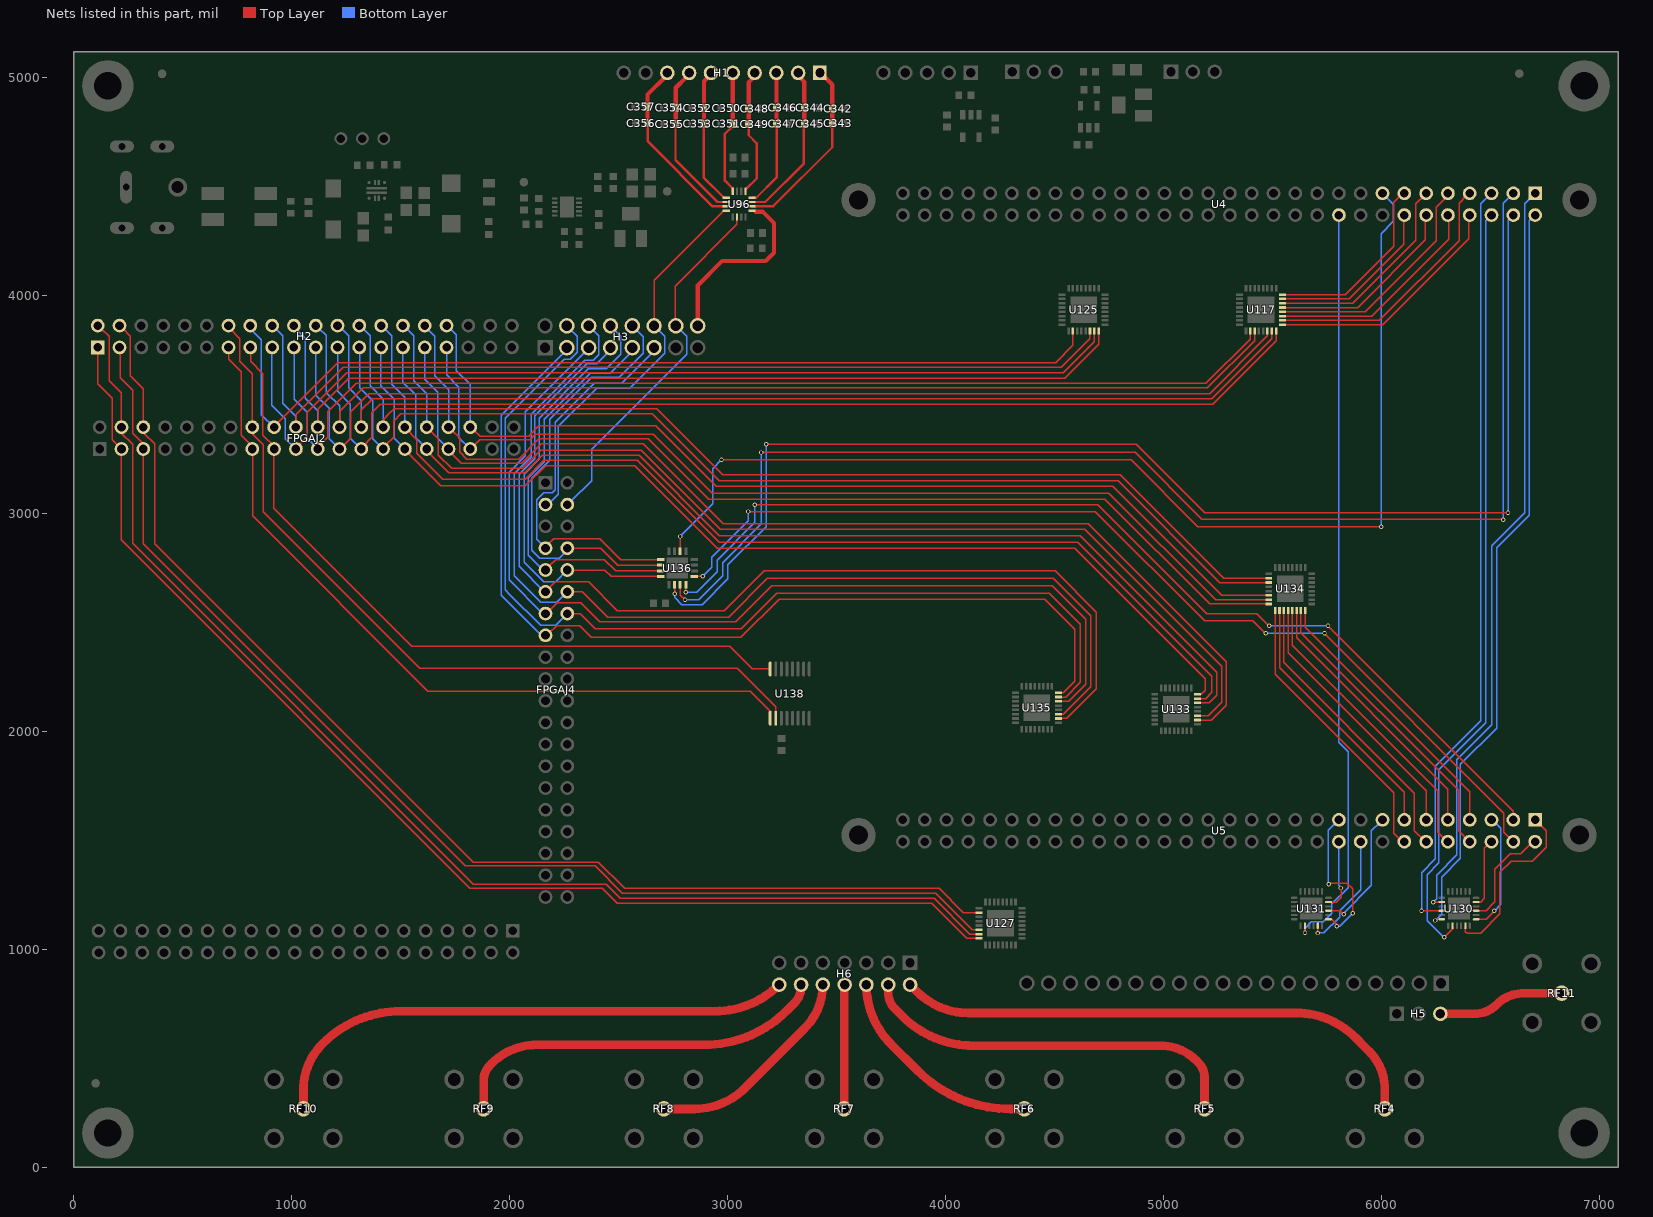
[diagram p0: the nets of this part, all layers, seen from the top]
# Altium PCB MISC82799.PcbDoc (part 2 of 5)
Units mil, origin at the board's own origin, x right, y up, seen from the top; angles counter-clockwise.
Board outline 7086.61 x 5118.11 mil, 4 copper layers (Top Layer, GND, POWER, Bottom Layer); 95 components, 232 nets, 857 pads, 1291 vias.

## Via types
v1: diameter 20, hole 12, Top Layer to Bottom Layer, 1291 vias

## Nets (pads, with @x,y where several pads share a name; then routed paths per layer and width w, separated by ;. In a path a pad name is that pad's centre, name@x,y a point inside that pad or via, vN(x,y) a via of type N, cw(c..) or ccw(c..) an arc to the next point about the centre after c; other vN are vias at no path point) (continued)
A_D_C4: U4.20 U131.8 | length 3458.9
  Top Layer w6: v1(5648.5,1075.5) U131.8@5648.5,1108.26
  Bottom Layer w6: v1@5649,1079 5649,1097 5678,1126 5732,1126 5772,1166 5772,1208 5847,1283 5847,1355 ; U4.20@5804.35,4367.81 5804.35,1949.65 5847,1907 5847,1355 ; 5847,1349 5847,1355
A_D_C5: U5.18 U131.11 | length 549.7
  Top Layer w6: v1(5707.5,1074.5) U131.11@5707.5,1108.26
  Bottom Layer w6: v1@5708,1075 5735,1075 5807,1147 5807,1177 5904.35,1274.35 U5.18@5904.35,1493.8
A_D_C6: U5.19 U131.13 | length 704.4
  Top Layer w6: U131.13@5756.74,1137.8 5772.2,1137.8 5794,1116 v1(5794,1105) ; v1@5760,1302 v1@5762,1304 ; v1@5761,1304 v1@5762,1304 ; v1(5868,1165) 5868,1277 5841,1304 v1@5762,1304
  Bottom Layer w6: v1(5757,1299) 5757,1302 5756,1303 5756,1457 5756,1545.45 5772.28,1561.72 U5.19@5804.35,1593.8 ; v1(5794,1105) 5808,1105 v1(5868,1165)
A_D_C7: U5.15 U131.15 | length 582.1
  Top Layer w6: U131.15@5756.94,1177 U131.15@5756.74,1177.2 5807.8,1177.2 v1@5824,1161
  Bottom Layer w6: v1(5826,1160) 5826,1166 5953,1293 5953,1543 U5.15@5993,1583 ; U5.15@5993.28,1582.72 U5.15@6004.35,1593.8
A_D_C8: U5.20 U131.17 | length 325.1
  Top Layer w6: U131.17@5756.74,1216.5 5791.5,1216.5 5814,1239 v1@5814,1288
  Bottom Layer w6: U5.20@5804.35,1493.8 5804.35,1293.65 v1@5811,1287
  other v1: 5813,1281
A_G_C1: U4.1 U130.2 | length 3484.7
  Top Layer w6: v1(6236.5,1216.5) U130.2@6276.26,1216.5
  Bottom Layer w6: v1@6236,1216 v1@6236,1219 ; v1@6238,1219 6252,1233 6252,1340 6345,1433 6345,1869 6505,2029 6505,2852 6656,3003 6656,4419.46 U4.1@6704.35,4467.81
A_G_C2: U4.5 U130.4 | length 3516.8
  Top Layer w6: v1(6183,1177) 6207.6,1177 6207.8,1177.2 U130.4@6276.26,1177.2
  Bottom Layer w6: v1@6184,1177 6184,1352 6247,1415 6247,1839 6456,2048 6456,4419.46 U4.5@6504.35,4467.81
A_G_C3: U4.2 U130.6 | length 3448.7
  Top Layer w6: v1@6249,1130 6256.8,1137.8 U130.6@6276.26,1137.8
  Bottom Layer w6: v1@6252,1137 6275,1160 6275,1331 6362,1418 6362,1848 6529,2015 6529,2841 6678,2990 6678,4341.46 U4.2@6704.35,4367.81
  other v1: 6247,1132
A_G_C4: U4.6 U130.8 | length 3537.7
  Top Layer w6: v1(6287,1055) 6325.5,1093.5 U130.8@6325.5,1108.26
  Bottom Layer w6: v1@6287,1054 6209,1132 6209,1343 6263,1397 6263,1824 6478,2039 6478,4341.46 U4.6@6504.35,4367.81
A_G_C5: U5.1 U130.11 | length 791
  Top Layer w6: U130.11@6384.5,1108.26 6384.5,1081.5 6392,1074 6455,1074 6543,1162 6543,1353 6595,1405 6692,1405 6755,1468 6755,1544 U5.1@6727,1572
A_G_C6: U5.5 U130.13 | length 524
  Top Layer w6: U130.13@6433.74,1137.8 6479.8,1137.8 v1@6516,1174
  Bottom Layer w6: v1@6518,1177 6547,1206 6547,1555 U5.5@6521,1581
  other v1: 6517,1177
A_G_C7: U5.2 U130.15 | length 476
  Top Layer w6: U130.15@6433.74,1177.2 U130.15@6445,1177.2 ; U130.15@6445,1177 6479,1177 6495.5,1193.5 6498.5,1196.5 6520,1218 6520,1367 6591,1438 6638,1438 U5.2@6692,1492
A_G_C8: U5.6 U130.17 | length 309.9
  Top Layer w6: U130.17@6433.74,1216.5 6454.5,1216.5 6471.5,1233.5 6471.5,1462.5 U5.6@6497,1488
A_N_R1: U4.4 U136.2 | length 5963.6
  Top Layer w6: v1(2757.2,2631.2) U136.2@2757.2,2672.23 ; v1(3177,3316) 4875,3316 5189,3002 v1(6580,3002)
  Bottom Layer w6: v1(2757.2,2631.2) 2757.2,2613.8 2790,2581 2883,2581 3002,2700 3002,2764 3177,2939 v1(3177,3316) ; v1(6580,3002) 6580,4343.46 U4.4@6604.35,4367.81
A_N_R2: U4.3 U136.3 | length 5983.9
  Top Layer w6: U136.3@2782.8,2672.23 2782.8,2625.2 v1(2805,2603) ; v1(3155,3279) 4869,3279 5176,2972 v1@6559,2972
  Bottom Layer w6: v1(2805,2603) 2825,2603 2867,2603 2977,2713 2977,2773 3155,2951 v1(3155,3279) ; v1(6558,2970) 6558,4421.46 U4.3@6604.35,4467.81
A_N_R3: U5.3 U136.4 | length 4698.2
  Top Layer w6: v1(2808.39,2637.39) U136.4@2808.39,2672.23 ; v1(3125,3039) 4698,3039 5198,2539 5428,2539 5483,2484 v1(5485,2484) ; v1(5754,2484) 6604.35,1633.65 U5.3@6604.35,1593.8
  Bottom Layer w6: v1(2808.39,2637.39) 2835,2637.39 2858.39,2637.39 2952,2731 2952,2785 3125,2958 v1(3125,3039) ; v1(5485,2484) v1(5754,2484)
A_N_R4: U5.4 U136.5 | length 4613.4
  Top Layer w6: U136.5@2846.77,2710.61 v1(2886.39,2710.61) ; v1(3095,3008) 4686,3008 5188,2506 5409,2506 5466,2449 v1(5469,2449) ; v1(5738,2449) 5737,2449 6561,1625 6561,1537.14 U5.4@6604.35,1493.8
  Bottom Layer w6: v1(2886.39,2710.61) 2906.89,2731.11 2928,2752.22 2928,2798 3095,2965 v1(3095,3008) ; v1(5469,2449) v1(5738,2449)
A_N_R5: U4.15 U136.10 | length 5222.8
  Top Layer w6: U136.10@2782.8,2825.77 v1(2782.8,2893.8) ; v1@2975,3245 4851,3245 5157,2939 v1(5999,2939)
  Bottom Layer w6: v1(2782.8,2893.8) 2932,3043 2932,3205 v1(2972,3245) ; v1@6000,2938 v1(5999,2939) 5998,2940 5998,4283 6054,4339 6054,4418.16 U4.15@6004.35,4467.81
A_S_R1: U4.8 U117.17 | length 1114.7
  Top Layer w6: U117.17@5545.42,3865.1 6006.1,3865.1 6400,4259 U4.8@6400,4356
A_S_R2: U4.7 U117.18 | length 1180.9
  Top Layer w6: U117.18@5545.42,3884.78 5989.78,3884.78 6356,4251 6356,4423 U4.7@6389,4456
A_S_R3: U4.10 U117.19 | length 1011.2
  Top Layer w6: U117.19@5545.42,3904.48 5955.48,3904.48 6307,4256 U4.10@6307,4360
A_S_R4: U4.9 U117.20 | length 1050.5
  Top Layer w6: U117.20@5545.42,3924.15 5924.16,3924.15 6251,4251 6251,4404 U4.9@6291,4444
A_S_R5: U4.12 U117.21 | length 883.5
  Top Layer w6: U117.21@5545.42,3943.85 5889.84,3943.85 6201,4255 U4.12@6201,4354
A_S_R6: U4.11 U117.22 | length 955
  Top Layer w6: U117.22@5545.42,3963.52 5867.52,3963.52 6157,4253 6157,4420 U4.11@6197,4460
A_S_R7: U4.14 U117.23 | length 782
  Top Layer w6: U117.23@5545.42,3983.22 5852.22,3983.22 6102,4233 U4.14@6102,4355
A_S_R8: U4.13 U117.24 | length 858.1
  Top Layer w6: U117.24@5545.42,4002.9 5832.9,4002.9 6056,4226 6056,4426 U4.13@6095,4465
A_W_R1: U5.7 U134.24 | length 1264.7
  Top Layer w6: U134.24@5650,2546 5650,2477 6404.35,1722.65 U5.7@6404.35,1593.8
A_W_R2: U5.8 U134.23 | length 1378.8
  Top Layer w6: U134.23@5630.22,2554.57 5630.22,2451.78 6353,1729 6353,1543 U5.8@6401,1495
A_W_R3: U5.9 U134.22 | length 1245.8
  Top Layer w6: U134.22@5610,2552 5610,2428 6304.35,1733.65 U5.9@6304.35,1593.8
A_W_R4: U5.10 U134.21 | length 1351.5
  Top Layer w6: U134.21@5590.84,2554.57 5590.84,2395.15 6258,1728 6258,1536 U5.10@6298,1496
A_W_R5: U5.11 U134.20 | length 1225.5
  Top Layer w6: U134.20@5571,2557 5571,2360 6204.35,1726.65 U5.11@6204.35,1593.8
A_W_R6: U5.12 U134.19 | length 1328.2
  Top Layer w6: U134.19@5551.48,2554.57 5551.48,2316.52 6151,1717 6151,1544 U5.12@6200,1495
A_W_R7: U5.13 U134.18 | length 1196.3
  Top Layer w6: U134.18@5532,2553 5532,2292 6104.35,1719.65 U5.13@6104.35,1593.8
A_W_R8: U5.14 U134.17 | length 1287.5
  Top Layer w6: U134.17@5512.1,2554.57 5512.1,2260.9 6055,1718 6055,1552 6055,1533 U5.14@6084,1504
BNC_DNW: H6.14 RF10.1 | length 2489.9
  Top Layer w40: RF10.1@1054.37,268 1054.37,354.04 cw(c1356.93,354.04) 1142.99,567.99 cw(c1500.32,210.66) 1500.32,716 2942.47,716 ccw(c2942.47,1132.53) H6.14@3237,838
BNC_DRAIN_1: H6.6 RF6.1 | length 1011.7
  Top Layer w40: H6.6@3637,838 ccw(c4023.27,838) 3750.14,564.86 3870.38,444.62 ccw(c4296.78,871.01) 4296.78,268 RF6.1@4361.46,268
BNC_DRAIN_2: H6.8 RF7.1 | length 589.2
  Top Layer w40: RF7.1@3534.68,268 ccw(c3529.1,273.59) 3537,273.59 cw(c3529.1,273.59) RF7.1@3534.68,268 ; RF7.1@3534.68,268 H6.8@3534.68,832.41 ; H6.8@3534.69,832.41 cw(c3542.59,832.41) H6.8@3537,838 ccw(c3542.59,832.41) H6.8@3534.69,832.41
BNC_GATE_1: H6.2 RF4.1 | length 2485.1
  Top Layer w40: H6.2@3837,838 3869.21,805.79 ccw(c4105.3,1041.89) 4105.3,708 5608.95,708 cw(c5608.95,326.43) 5878.76,596.24 5926,549 5942.48,532.52 ; 5942.48,532.53 cw(c5767.38,357.43) 6015,357.43 RF4.1@6015,268
BNC_GATE_2: H6.4 RF5.1 | length 1803.5
  Top Layer w40: H6.4@3737,838 3737,799.42 ccw(c3837,799.42) 3766.29,728.71 3802.22,692.78 ccw(c4127.61,1018.18) 4127.61,558 4986.7,558 cw(c4986.7,327.92) 5149.39,490.61 5158.94,481.06 cw(c5088.23,410.35) 5188.23,410.35 RF5.1@5188.23,268
BNC_PSUB: H5.3 RF11.1 | length 578.4
  Top Layer w40: H5.3@6270,704 6425.18,704 ccw(c6425.18,848.43) 6527.3,746.3 cw(c6654.53,619.08) 6654.53,799 RF11.1@6823,799
BNC_SOURCE: H6.10 RF8.1 | length 1007.6
  Top Layer w40: RF8.1@2707.91,268 2849.47,268 ccw(c2849.47,592.78) 3079.13,363.13 3354.27,638.27 ccw(c3154.54,838) H6.10@3437,838
BNC_WELL: H6.12 RF9.1 | length 1779.8
  Top Layer w40: RF9.1@1881.14,268 1881.14,397.72 cw(c1981.14,397.72) 1910.43,468.43 1918.76,476.76 cw(c2124.54,270.98) 2124.54,562 2894.55,562 ccw(c2894.55,1094.2) 3270.88,717.88 3307.71,754.71 ccw(c3237,825.42) 3337,825.42 H6.12@3337,838
CTRL_DNW_A0: FPGAJ4.9 H3.9 U136.15 | length 1834.7
  Top Layer w6: FPGAJ4.9@2179,2756 2211,2788 2435,2788 2486.8,2736.2 U136.15@2693.23,2736.2
  Bottom Layer w6: FPGAJ4.9@2165,2740 2152,2740 2085,2807 2085,3163 2159,3237 2159,3431 2370,3642 2462,3642 H3.9@2556,3736
CTRL_DNW_A1: FPGAJ4.8 H3.10 U136.14 | length 1976.2
  Top Layer w6: FPGAJ4.8@2273,2839 2419,2839 2496.2,2761.8 U136.14@2693.23,2761.8
  Bottom Layer w6: FPGAJ4.8@2260,2826 2227,2793 2139,2793 2102,2830 2102,3160 2185,3243 2185,3432 2378,3625 2504,3625 2614,3735 2614,3809 H3.10@2563,3860
CTRL_DNW_A2: FPGAJ4.7 H3.11 U136.13 | length 1801.4
  Top Layer w6: FPGAJ4.7@2174,2855 2203,2884 2413,2884 2509.61,2787.39 U136.13@2693.23,2787.39
  Bottom Layer w6: FPGAJ4.7@2165,2840 2124,2881 2124,3061 2157,3094 2197,3094 2210,3107 2210,3418 2389,3597 2514,3597 H3.11@2654,3737
CTRL_DNW_EN: FPGAJ4.10 H3.8 U136.16 | length 2091.3
  Top Layer w6: FPGAJ4.10@2289,2739 2424,2739 ; 2322,2739 2424,2739 ; U136.16@2693.23,2710.61 2465.39,2710.61 2437,2739 2424,2739
  Bottom Layer w6: FPGAJ4.10@2265,2740 2212,2687 2156,2687 2067,2776 2067,3180 2137,3250 2137,3437 2362,3662 2444,3662 2511,3729 2511,3811 H3.8@2476,3846
CTRL_GD_A0_BOTTOM: FPGAJ2.15 H2.13 U138.1 | length 3590
  Top Layer w6: H2.13@713,3746 713,3707 770,3650 770,3357 820,3307 FPGAJ2.15@820,3295 ; 821,3253 821,3230 ; FPGAJ2.15@821,3282 821,3230 ; U138.1@3195.43,2060.18 3195.43,2092.57 3104,2184 1625,2184 821,2988 821,3230
CTRL_GD_A0_LEFT: FPGAJ2.19 H2.17 U125.15 | length 4472.4
  Top Layer w6: FPGAJ2.19@1024,3306 1072,3354 1072,3464 1253,3645 4540.22,3645 4673.11,3777.89 ; 4673,3778 4682.22,3787.22 U125.15@4682.22,3835.57
  Bottom Layer w6: H2.17@909,3751 909,3496 972,3433 972,3343 FPGAJ2.19@1020,3295
CTRL_GD_A0_RIGHT: FPGAJ2.4 H2.2 U127.15 | length 5665.3
  Top Layer w6: H2.2@130,3844 163,3811 163,3609 220,3552 FPGAJ2.4@220,3395 220,3368 271,3317 271,2862 1834,1299 2443,1299 2508,1234 3947,1234 4111.22,1069.78 U127.15@4153.58,1069.78
CTRL_GD_A1_BOTTOM: FPGAJ2.17 H2.15 U138.16 | length 3334.5
  Top Layer w6: H2.15@812,3741 812,3697 869,3640 869,3358 920,3307 FPGAJ2.17@920,3295 ; 918,3248 918,3240 ; FPGAJ2.17@918,3276 918,3240 ; U138.16@3195.43,2285.82 3114.17,2285.82 3010,2390 1551,2390 918,3023 918,3240
CTRL_GD_A1_LEFT: FPGAJ2.20 H2.18 U125.14 | length 4361.4
  Top Layer w6: FPGAJ2.20@1020.48,3401.48 1020.48,3453.48 1237,3670 4531,3670 4662.52,3801.52 U125.14@4662.52,3835.57
  Bottom Layer w6: H2.18@928,3846 960,3814 960,3505 1020,3445 FPGAJ2.20@1020,3395
CTRL_GD_A1_RIGHT: FPGAJ2.5 H2.3 U127.14 | length 5513.9
  Top Layer w6: H2.3@214,3750 214,3621 271,3564 271,3367 320,3318 FPGAJ2.5@320,3295 ; 319,3253 319,3229 ; FPGAJ2.5@319,3283 319,3229 ; U127.14@4153.58,1089.48 4123.52,1089.48 3956,1257 2518,1257 2392,1383 1796,1383 319,2860 319,3229
CTRL_GD_A2_LEFT: FPGAJ2.18 H2.16 U125.10 | length 4364.8
  Top Layer w6: FPGAJ2.18@927,3406 951,3430 ; 948,3427 951,3430 ; U125.10@4583.78,3829 U125.10@4583.78,3835.57 ; U125.10@4584,3829 4584,3770 4505,3691 1212,3691 951,3430
  Bottom Layer w6: H2.16@818,3840 862,3796 862,3453 FPGAJ2.18@920,3395
CTRL_GD_A2_RIGHT: FPGAJ2.6 H2.4 U127.10 | length 5518.6
  Top Layer w6: H2.4@225,3848 260,3813 260,3632 320,3572 FPGAJ2.6@320,3395 ; FPGAJ2.6@325,3385 325,3365 372,3318 372,2861 1833.5,1399.5 2407.5,1399.5 2528,1279 3970,1279 4080.78,1168.22 U127.10@4153.58,1168.22
CTRL_GD_EN_BOTTOM: FPGAJ2.16 H2.14 U138.2 | length 3673.5
  Top Layer w6: H2.14@718,3846 763,3801 763,3697 820,3640 FPGAJ2.16@820,3395 ; FPGAJ2.16@821,3394 821,3363 870,3314 870,3008 1589,2289 3044,2289 3221.02,2111.98 U138.2@3221.02,2060.18
CTRL_GD_EN_LEFT: FPGAJ2.22 H2.20 U125.16 | length 4351.9
  Top Layer w6: FPGAJ2.22@1122,3406 1123,3407 1123,3470 ; 1123,3440 1123,3470 ; U125.16@4701.9,3835.57 4701.9,3774.9 4546,3619 1262,3619 1123,3480 1123,3470
  Bottom Layer w6: H2.20@1024,3841 1062,3803 1062,3528 1120,3470 FPGAJ2.22@1120,3395
CTRL_GD_EN_RIGHT: FPGAJ2.3 H2.1 U127.16 | length 5600.3
  Top Layer w6: H2.1@111,3743 111,3594 177,3528 177,3358 177,3338 FPGAJ2.3@220,3295 220,2879 1818.5,1280.5 2425.5,1280.5 2495,1211 3936,1211 4096.9,1050.1 U127.16@4153.58,1050.1
CTRL_SOURCE_A0_LEFT: FPGAJ2.26 H2.24 U117.15 | length 4910.5
  Top Layer w6: FPGAJ2.26@1320,3411 1320,3474 1372,3526 2995,3526 ; 2989,3526 2995,3526 ; U117.15@5496.22,3835.57 5496.22,3801.22 5221,3526 2995,3526
  Bottom Layer w6: H2.24@1225,3851 1262,3814 1262,3575 1320,3517 FPGAJ2.26@1320,3395
CTRL_SOURCE_A0_RIGHT: FPGAJ2.30 H2.28 U133.15 | length 4925.2
  Top Layer w6: FPGAJ2.30@1523,3389 1574,3338 1574,3276 1693,3157 2071,3157 2158,3244 2585,3244 2961,2868 4607,2868 5222,2253 5222,2178 5194.22,2150.22 U133.15@5156.42,2150.22
  Bottom Layer w6: H2.28@1423,3850 1459,3814 1459,3593 1520,3532 FPGAJ2.30@1520,3395
CTRL_SOURCE_A1_LEFT: FPGAJ2.23 H2.21 U117.14 | length 5059.5
  Top Layer w6: FPGAJ2.23@1228,3301 1271,3344 1271,3466 1354,3549 5211,3549 5476.52,3814.52 U117.14@5476.52,3835.57
  Bottom Layer w6: H2.21@1112,3756 1112,3542 1173,3481 1173,3342 FPGAJ2.23@1220,3295
CTRL_SOURCE_A1_RIGHT: FPGAJ2.31 H2.29 U133.14 | length 4821.6
  Top Layer w6: FPGAJ2.31@1628,3279 1721,3186 2070,3186 2150,3266 2257,3266 ; 2252,3266 2257,3266 ; 3054,2898 3059,2898 ; U133.14@5156.42,2130.52 5210.52,2130.52 5245,2165 5245,2270 4617,2898 3059,2898 ; 2257,3266 2594,3266 2962,2898 3059,2898
  Bottom Layer w6: H2.29@1510,3752 1510,3602 1569,3543 1569,3346 FPGAJ2.31@1620,3295
CTRL_SOURCE_A2_LEFT: FPGAJ2.24 H2.22 U117.11 | length 4951.6
  Top Layer w6: FPGAJ2.24@1221,3402 1221,3457 ; 1221,3435.5 1221,3457 ; U117.11@5417.48,3835.57 5417.48,3792.48 5201,3576 1329,3576 1221,3468 1221,3457
  Bottom Layer w6: H2.22@1128,3847 1159,3816 1159,3554 1220,3493 FPGAJ2.24@1220,3395
CTRL_SOURCE_A2_RIGHT: FPGAJ2.32 H2.30 U133.11 | length 4996.7
  Top Layer w6: FPGAJ2.32@1634,3382 1674,3342 1674,3267 1734,3207 2061,3207 2144,3290 2603,3290 2967,2926 3061,2926 ; 3051,2926 3061,2926 ; U133.11@5156.42,2071.48 5204.48,2071.48 5266,2133 5266,2298 4638,2926 3061,2926
  Bottom Layer w6: H2.30@1526,3849 1560,3815 1560,3608 1620,3548 FPGAJ2.32@1620,3395
CTRL_SOURCE_A3_LEFT: FPGAJ2.21 H2.19 U117.10 | length 5067.4
  Top Layer w6: FPGAJ2.21@1128,3310 1166,3348 1166,3465 1297,3596 5194,3596 5397,3799 U117.10@5397,3831 ; U117.10@5397.78,3831 U117.10@5397.78,3835.57
  Bottom Layer w6: H2.19@1012,3741 1012,3522 1071,3463 1071,3344 FPGAJ2.21@1120,3295
CTRL_SOURCE_A3_RIGHT: FPGAJ2.33 H2.31 U133.10 | length 4906
  Top Layer w6: FPGAJ2.33@1725,3283 1779,3229 2056,3229 2145,3318 2614,3318 2980,2952 3053,2952 ; 3049,2952 3053,2952 ; U133.10@5156.42,2051.78 5219.78,2051.78 5288,2120 5288,2319 4655,2952 3053,2952
  Bottom Layer w6: H2.31@1611,3757 1611,3615 1671,3555 1671,3344 FPGAJ2.33@1720,3295
CTRL_SOURCE_EN_LEFT: FPGAJ2.25 H2.23 U117.16 | length 5009.8
  Top Layer w6: FPGAJ2.25@1326,3306 1368,3348 1368,3461 1408,3501 3002,3501 ; 2993,3501 3002,3501 ; U117.16@5515.9,3835.57 5515.9,3790.9 5226,3501 3002,3501
  Bottom Layer w6: H2.23@1211,3749 1211,3560 1270,3501 1270,3345 FPGAJ2.25@1320,3295
CTRL_SOURCE_EN_RIGHT: FPGAJ2.29 H2.27 U133.16 | length 4769.9
  Top Layer w6: FPGAJ2.29@1521,3287 1523,3287 1684,3126 2073,3126 2165,3218 2574,3218 2953,2839 4593,2839 5192,2240 5192,2188 5173.9,2169.9 U133.16@5156.42,2169.9
  Bottom Layer w6: H2.27@1409,3743 1409,3586 1471,3524 1471,3344 FPGAJ2.29@1520,3295
CTRL_WELL_A0_LEFT: FPGAJ2.35 H2.33 U134.15 | length 4510.1
  Top Layer w6: FPGAJ2.35@1828,3303 1863,3338 2094,3338 2119,3363 2660,3363 2930,3093 2982,3093 ; 2966,3093 2982,3093 ; U134.15@5482.58,2603.78 5238.22,2603.78 4749,3093 2982,3093
  Bottom Layer w6: H2.33@1711,3750 1711,3636 1768,3579 1768,3347 FPGAJ2.35@1820,3295
CTRL_WELL_A0_RIGHT: FPGAJ4.14 H3.4 U135.15 | length 4644.9
  Top Layer w6: FPGAJ4.14@2272,2540 2324,2540 2394,2470 3063,2470 3226,2633 4475,2633 4618,2490 4618,2224 4551.22,2157.22 U135.15@4517.42,2157.22
  Bottom Layer w6: FPGAJ4.14@2265,2540 2211,2486 2142,2486 2002,2626 1979.5,2648.5 1979.5,3436.5 2250,3707 2278,3707 2310,3739 2310,3811 H3.4@2269,3852
CTRL_WELL_A1_LEFT: FPGAJ2.36 H2.34 U134.14 | length 4504.3
  Top Layer w6: FPGAJ2.36@1836,3382 1865,3353 1890,3353 2087,3353 2135,3401 2670,3401 2948,3123 2973,3123 ; 2966,3123 2973,3123 ; U134.14@5482.58,2623.48 5266.52,2623.48 4767,3123 2973,3123
  Bottom Layer w6: H2.34@1724,3852 1756,3820 1756,3655 1820,3591 FPGAJ2.36@1820,3395
CTRL_WELL_A1_RIGHT: FPGAJ4.13 H3.5 U135.14 | length 4552
  Top Layer w6: FPGAJ4.13@2173,2544 2218,2589 2327,2589 2414,2502 3038,2502 3203,2667 4489,2667 4642,2514 4642,2215 4564.52,2137.52 U135.14@4517.42,2137.52
  Bottom Layer w6: FPGAJ4.13@2153,2540 1998,2695 1998,3188 2073,3263 2073,3466 2362,3755 H3.5@2362,3766
CTRL_WELL_A2_LEFT: FPGAJ2.27 H2.25 U134.11 | length 4976.7
  Top Layer w6: FPGAJ2.27@1433,3314 1468,3349 1468,3366 1468,3423 1502,3457 2655,3457 2963,3149 4792,3149 5258.48,2682.52 U134.11@5482.58,2682.52
  Bottom Layer w6: H2.25@1312,3754 1312,3577 1372,3517 1372,3343 FPGAJ2.27@1420,3295
CTRL_WELL_A2_RIGHT: FPGAJ4.12 H3.6 U135.11 | length 4758.7
  Top Layer w6: FPGAJ4.12@2275,2640 2334,2640 2450,2524 3006,2524 3183,2701 4495,2701 4667,2529 4667,2205 4540.48,2078.48 U135.11@4517.42,2078.48
  Bottom Layer w6: FPGAJ4.12@2265,2640 2216,2591 2143,2591 2021,2713 2021,3181 2099,3259 2099,3454 2346,3701 2383,3701 2410,3728 2410,3814 H3.6@2375,3849
CTRL_WELL_A3_LEFT: FPGAJ2.28 H2.26 U134.10 | length 4939.1
  Top Layer w6: FPGAJ2.28@1422,3403 1422,3431 1447,3456 ; 1437,3446 1447,3456 ; U134.10@5482.58,2702.22 5276.78,2702.22 4802,3177 2977,3177 2675,3479 1470,3479 1447,3456
  Bottom Layer w6: H2.26@1324,3850 1360,3814 1360,3584 1420,3524 FPGAJ2.28@1420,3395
CTRL_WELL_A3_RIGHT: FPGAJ4.11 H3.7 U135.10 | length 4689
  Top Layer w6: FPGAJ4.11@2176,2652 2209,2685 2363,2685 2495,2553 2985,2553 3168,2736 4503,2736 4692,2547 4692,2196 4554.78,2058.78 U135.10@4517.42,2058.78
  Bottom Layer w6: FPGAJ4.11@2160,2641 2044,2757 2044,3179 2116,3251 2116,3447 2354,3685 2401,3685 2463,3747 H3.7@2463,3760
CTRL_WELL_EN_LEFT: FPGAJ2.34 H2.32 U134.16 | length 4713.8
  Top Layer w6: FPGAJ2.34@1736,3381 1771,3346 1771,3282 1804,3249 2043,3249 2135,3341 2636,3341 2913,3064 2998,3064 ; 2970,3064 2998,3064 ; U134.16@5482.58,2584.1 5210.9,2584.1 4731,3064 2998,3064
  Bottom Layer w6: H2.32@1620,3849 1657,3812 1657,3630 1720,3567 FPGAJ2.34@1720,3395
CTRL_WELL_EN_RIGHT: FPGAJ4.15 H3.3 U135.16 | length 4434.7
  Top Layer w6: FPGAJ4.15@2182,2451 2216,2485 2321,2485 2375,2431 3061,2431 3236,2606 4456,2606 4593,2469 4593,2229 4540.9,2176.9 U135.16@4517.42,2176.9
  Bottom Layer w6: FPGAJ4.15@2165,2440 2145,2440 1962,2623 1962,3450 H3.3@2254,3742 ; H3.3@2256.5,3739.5 H3.3@2258,3741
DAC0: C342.2 C343.2 H1.1 U96.2 | length 814.2
  Top Layer w11: U96.2@3112.06,4408.16 3209.16,4408.16 3480,4679 C343.2@3480,4786
  Top Layer w20: H1.1@3446,5001 3480.83,4966.17 C343.2@3480.83,4788.31
DAC1: C344.2 C345.2 H1.2 U96.3 | length 714.7
  Top Layer w11: U96.3@3112.06,4427.84 3172.84,4427.84 3350,4605 C345.2@3350,4784
  Top Layer w20: H1.2@3330,5001 3352.59,4978.41 C344.2@3352.59,4860 C345.2@3352.59,4786
DAC2: C346.2 C347.2 H1.3 U96.4 | length 613.3
  Top Layer w11: U96.4@3112.06,4447.53 3131.53,4447.53 3225,4541 C347.2@3225,4779
  Top Layer w20: C347.2@3224.59,4786 H1.3@3224.59,5009.59
DAC3: C348.2 C349.2 H1.4 U96.5 | length 576
  Top Layer w11: U96.5@3082.53,4477.05 3082.53,4484.53 3134,4536 3134,4697 3097,4734 C349.2@3097,4779
  Top Layer w20: C349.2@3096.59,4785 3096.59,4976.59 H1.4@3129,5009
DAC4: C350.2 C351.2 H1.5 U96.8 | length 542
  Top Layer w11: C351.2@3022,4775 2988,4741 2988,4526 3023.48,4490.52 U96.8@3023.48,4477.05
  Top Layer w20: C351.2@3023.71,4786 C350.2@3023.71,4858 H1.5@3023.71,5001.29
DAC5: C352.2 C353.2 H1.6 U96.9 | length 611.1
  Top Layer w11: C353.2@2890,4785 2890,4541 2983.47,4447.53 U96.9@2993.95,4447.53
  Top Layer w20: C353.2@2891.71,4786 2891.71,4981.71 H1.6@2912,5002
DAC6: C354.2 C355.2 H1.7 U96.10 | length 718.5
  Top Layer w11: C355.2@2761,4793 2761,4621 2954.16,4427.84 U96.10@2993.95,4427.84
  Top Layer w20: C355.2@2762.71,4785 2762.71,4951.71 H1.7@2810,4999
DAC7: C356.2 C357.2 H1.8 U96.11 | length 816.8
  Top Layer w12: C356.2@2634,4791 2634,4706 2931.84,4408.16 U96.11@2993.95,4408.16
  Top Layer w20: C356.2@2632.71,4790 2632.71,4920.71 H1.8@2716,5004
DAC_CS: FPGAJ4.3 H3.12 U96.12 | length 1853.1
  Top Layer w6: H3.12@2664,3876 2664,3969 ; 2664,3911 2664,3969 ; U96.12@2993.95,4388.47 2982.47,4388.47 2664,4070 2664,3969
  Bottom Layer w6: FPGAJ4.3@2185,3049 2224.5,3088.5 2224.5,3398.5 2400,3574 2552,3574 2712,3734 2712,3813 H3.12@2678,3847 ; H3.12@2663,3860 H3.12@2677,3846
DAC_REF: H3.16 U96.1 | length 856
  Top Layer w6: U96.1@3112.06,4388.47 3129,4388.47
  Top Layer w20: H3.16@2863,3860 2863,4045 2975,4157 3175,4157 3213,4195 3213,4331 3160,4384 3129,4384
DAC_SDI: FPGAJ4.4 H3.14 U96.14 | length 1631.5
  Top Layer w6: H3.14@2760,3890 2760,4042 3043.16,4325.16 U96.14@3043.16,4358.94
  Bottom Layer w6: FPGAJ4.4@2281,3055 2376,3150 2376,3293 2812,3729 2812,3811 H3.14@2763,3860